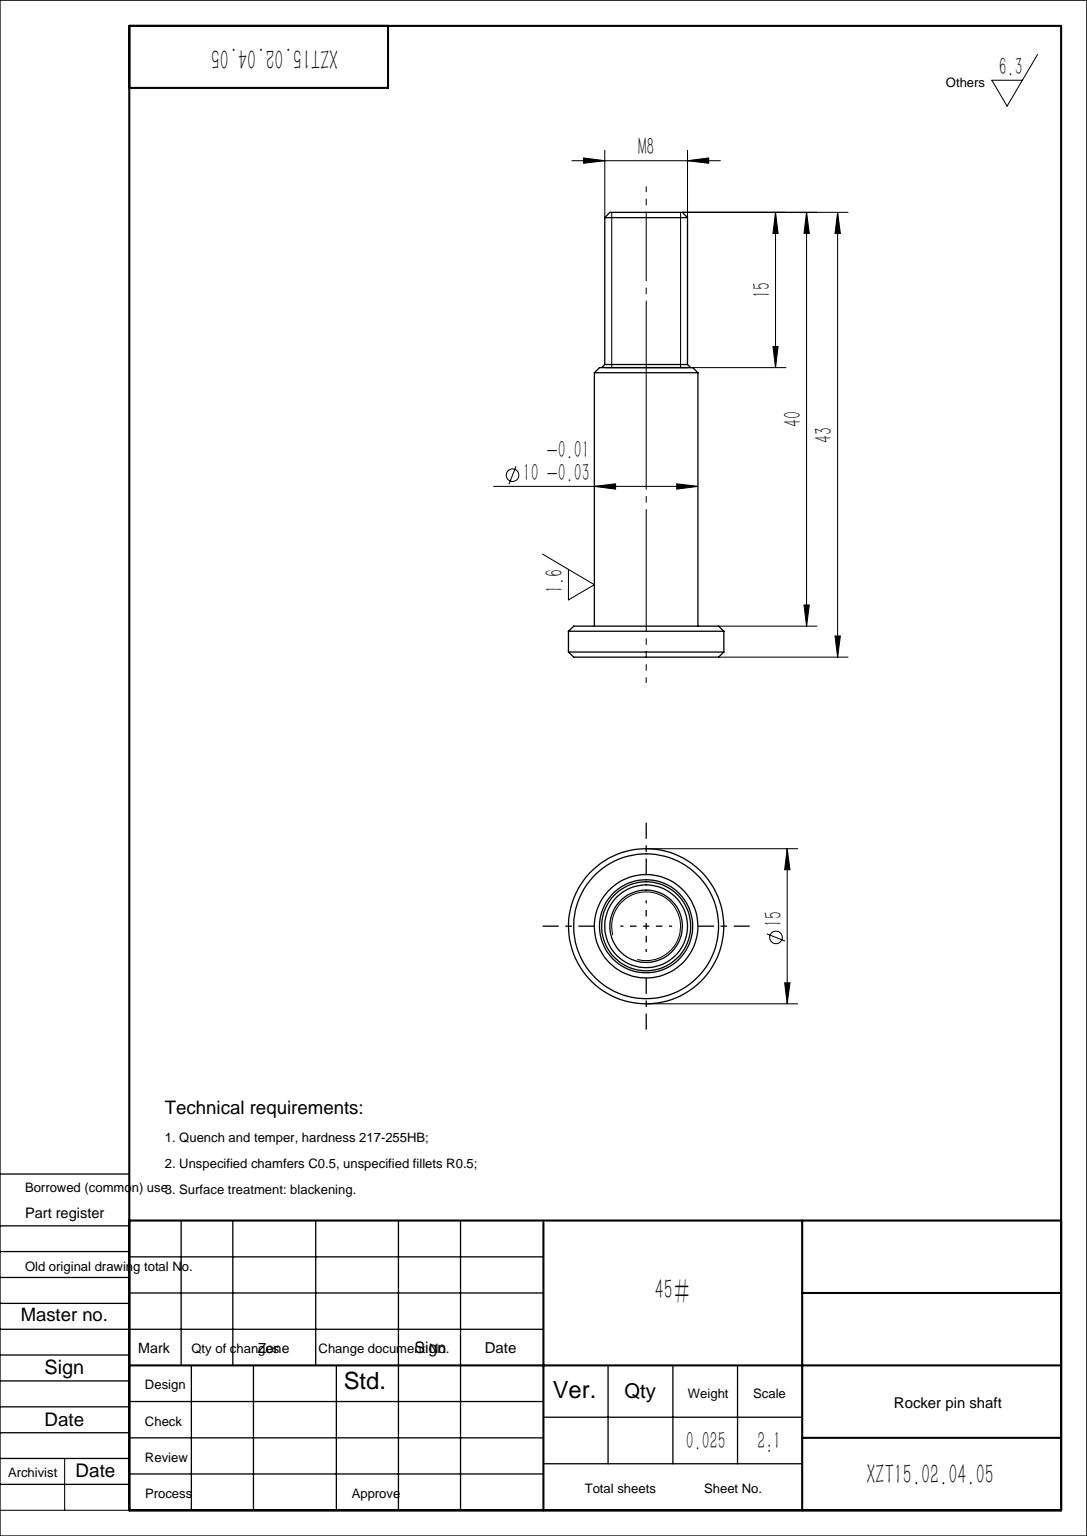
SolidWorks part; units mm, degrees
material "45#"
ref_plane "Front Plane" through (0, 0, 0) normal (0, 0, 1) x (1, 0, 0)
ref_plane "Top Plane" through (0, 0, 0) normal (0, 1, 0) x (1, 0, 0)
ref_plane "Right Plane" through (0, 0, 0) normal (1, 0, 0) x (0, 0, -1)
sketch "Sketch1" plane through (0, 0, 0) normal (0, 0, 1) x (1, 0, 0)
  line L0 (0, 0) -> (7.5, 0)
  line L1 (7.5, 0) -> (7.5, 3)
  line L2 (7.5, 3) -> (5, 3)
  line L3 (5, 3) -> (5, 28)
  line L4 (5, 28) -> (4, 28)
  line L5 (4, 28) -> (4, 43)
  line L6 (4, 43) -> (0, 43)
  line L7 (0, 43) -> (0, 0)
  line L8 (0, 0) -> (0, -4.6727) construction
  dimension "D1" = 15
  dimension "D2" = 10
  dimension "D3" = 8
  dimension "D4" = 15
  dimension "D5" = 40
  dimension "D6" = 43
revolve "Revolve1" add sketch "Sketch1" angle 360 about L8
cosmetic thread "Cosmetic Thread1"
chamfer "Chamfer1" distance 0.5 angle 45 4 edges at (0, 43, 4) (0, 0, 7.5) (0, 28, 5) (0, 3, 7.5)
chamfer "Chamfer2" distance 0.3 angle 45 1 edges at (0, 28, 4)
